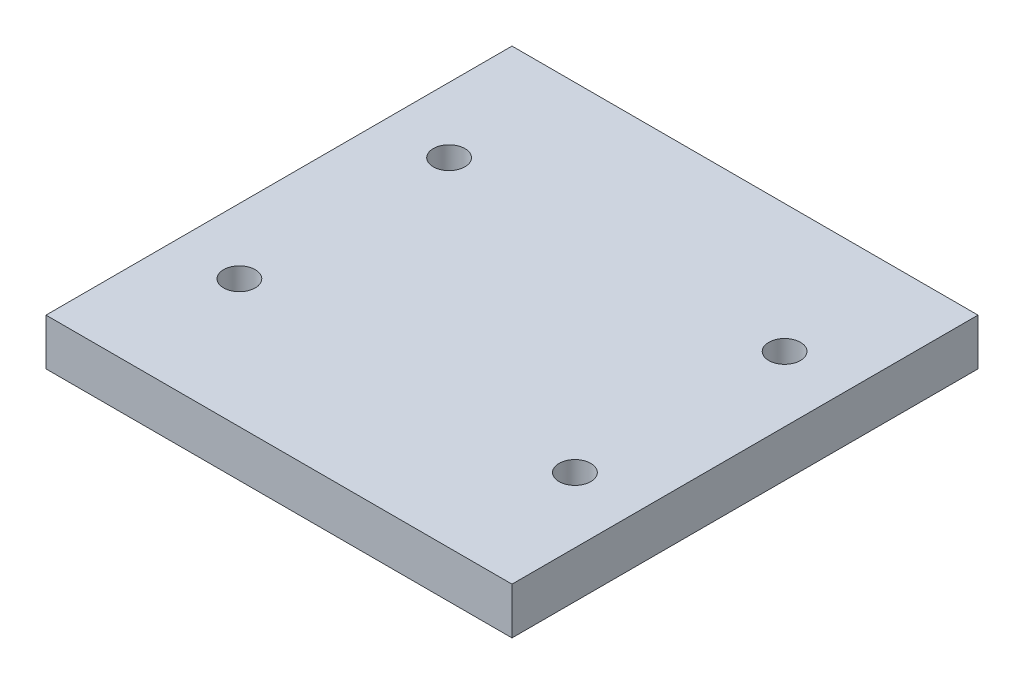
SolidWorks part; units mm, degrees
ref_plane "前视基准面" through (0, 0, 0) normal (0, 0, 1) x (1, 0, 0)
ref_plane "上视基准面" through (0, 0, 0) normal (0, 1, 0) x (1, 0, 0)
ref_plane "右视基准面" through (0, 0, 0) normal (1, 0, 0) x (0, 0, -1)
sketch "草图1" plane through (0, 0, 0) normal (0, 1, 0) x (1, 0, 0)
  line L0 (0, 0) -> (0, 69.4728) construction
  line L1 (-50, 50) -> (50, 50)
  line L2 (-50, 50) -> (-50, -50)
  line L3 (-50, -50) -> (50, -50)
  line L4 (50, 50) -> (50, -50)
  line L5 (0, 0) -> (68.8287, 0) construction
  dimension "D1" = 100
  dimension "D2" = 100
  dimension "D3" = 50
  dimension "D4" = 50
extrude "拉伸1" add sketch "草图1" along normal blind 10
hole_wizard "M8 螺纹孔1" positions "3D草图1" profile "草图3" tap size "M8" standard "ISO" end condition through all
sketch3d "3D草图1"
  line L4 (-50, 0, 0) -> (50, 0, 0) construction
  line L5 (-50, 0, -50) -> (-50, 0, 50) construction
  line L6 (50, 0, 50) -> (50, 0, -50) construction
  line L8 (0, 0, 50) -> (0, 0, -50) construction
  line L9 (-50, 0, 50) -> (50, 0, 50) construction
  line L10 (50, 0, -50) -> (-50, 0, -50) construction
  point P0 (-36, 0, 22.5)
  point P2 (-36, 0, -22.5)
  point P4 (36, 0, 22.5)
  point P6 (36, 0, -22.5)
  dimension "D1" = 22.5
  dimension "D2" = 22.5
  dimension "D3" = 36
  dimension "D4" = 36
sketch "草图3" plane through (-36, 0, 22.5) normal (1, 0, 0) x (0, 0, -1)
  line L0 (0, 0) -> (0, 10)
  line L1 (0, 10) -> (3.4, 10)
  line L2 (3.4, 10) -> (3.4, 0)
  line L5 (3.4, 0) -> (0, 0)
  line L11 (0, -6.35) -> (0, 107.95) construction
  dimension "通孔螺纹孔钻头直径" = 6.8
  dimension "通孔螺纹孔钻头深度" = 10
cosmetic thread "孔螺蚊线1" parameters "D2"=8
cosmetic thread "孔螺蚊线2" parameters "D2"=8
cosmetic thread "孔螺蚊线3" parameters "D2"=8
cosmetic thread "孔螺蚊线4" parameters "D2"=8
